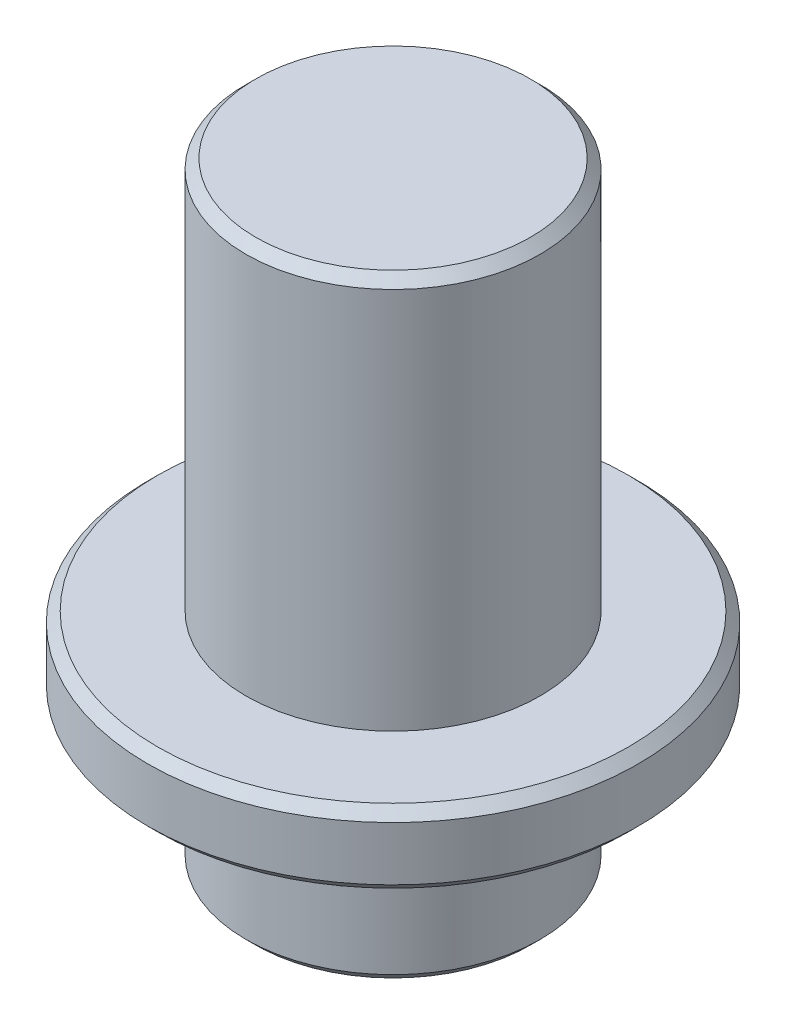
from build123d import *

# Parameters (mm, degrees)
SKETCH1_R           = 5
BOSS_EXTRUDE1_DEPTH = 1.5
SKETCH2_R           = 3
BOSS_EXTRUDE2_DEPTH = 8
BOSS_EXTRUDE3_START = 3
SKETCH3_R           = 3
BOSS_EXTRUDE3_DEPTH = 3
CHAMFER1_SIZE       = 0.2


with BuildPart() as part:
    # Sketch1 → Boss-Extrude1 (new body)
    with BuildSketch(Plane(origin=(0, 0, 0), x_dir=(1, 0, 0), z_dir=(0, 1, 0))):
        with Locations(Location((0, 0, 0), (0, 0, 270))):
            Circle(SKETCH1_R)
    extrude(amount=BOSS_EXTRUDE1_DEPTH)

    # Sketch2 → Boss-Extrude2 (add)
    with BuildSketch(Plane(origin=(0, 1.5, 0), x_dir=(1, 0, 0), z_dir=(0, 1, 0))):
        with Locations(Location((0, 0, 0), (0, 0, 270))):
            Circle(SKETCH2_R)
    extrude(amount=BOSS_EXTRUDE2_DEPTH)

    # Sketch3 → Boss-Extrude3 (add)
    with BuildSketch(Plane.XZ.offset(BOSS_EXTRUDE3_START)):
        with Locations(Location((0, 0, 0), (0, 0, 90))):
            Circle(SKETCH3_R)
    extrude(amount=-BOSS_EXTRUDE3_DEPTH)

    # Chamfer1
    chamfer1_edges = [part.edges().sort_by_distance(p)[0] for p in [
        (0, -3, -3),
        (0, 0, -5),
        (0, 1.5, -5),
        (0, 9.5, -3),
    ]]
    chamfer(chamfer1_edges, length=CHAMFER1_SIZE)


solid = part.part
